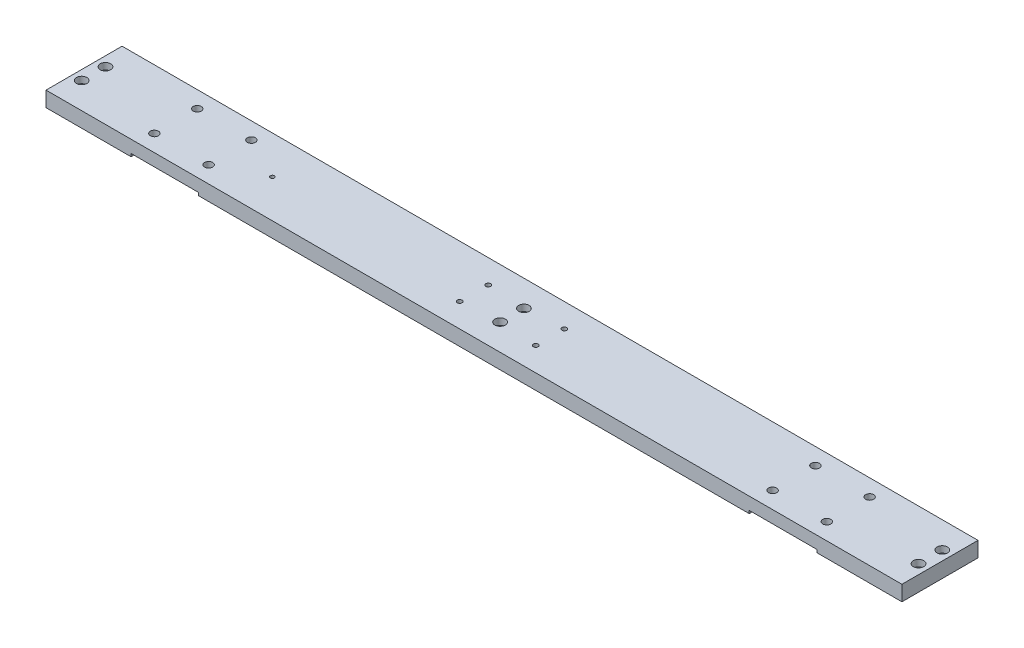
from build123d import *

# Parameters (mm, degrees)
SKETCH_1_W                = 900
SKETCH_1_H                = 80
EXTRUDE_1_DEPTH           = 16
SKETCH_2_W                = 71.098057304
SKETCH_2_H                = 80
CUT_EXTRUDE_1_DEPTH       = 3
HOLE_WIZARD_8_5_8_5_1_D   = 8.5
HOLE_WIZARD_M6_1_D        = 5
HOLE_WIZARD_1_D           = 6.6
HOLE_WIZARD_1_CBORE_D     = 11
HOLE_WIZARD_1_CBORE_DEPTH = 6.8
PATTERN_LINEAR_1_COUNT    = 3
PATTERN_LINEAR_1_PITCH    = 440
HOLE_WIZARD_M5_1_D        = 4.2


with BuildPart() as part:
    # 草图1 → 凸台-拉伸1 (new body)
    with BuildSketch(Plane(origin=(0, 0, 0), x_dir=(1, 0, 0), z_dir=(0, 1, 0))):
        Rectangle(SKETCH_1_W, SKETCH_1_H)
    extrude(amount=EXTRUDE_1_DEPTH)

    # 草图2 → 切除-拉伸1 (cut)
    with BuildSketch(Plane.XZ):
        with Locations((-325, 0)):
            Rectangle(SKETCH_2_W, SKETCH_2_H)
        with Locations((325, 0)):
            Rectangle(SKETCH_2_W, SKETCH_2_H)
    extrude(amount=-CUT_EXTRUDE_1_DEPTH, mode=Mode.SUBTRACT)

    # Ø8.5 (8.5) 直径孔1 (through all)
    with Locations(Plane(origin=(0, 16, 0), x_dir=(1, 0, 0), z_dir=(0, 1, 0))):
        with Locations((-353.5, 22.5), (-296.5, 22.5), (-353.5, -22.5), (-296.5, -22.5)):
            hole_wizard_8_5_8_5_1 = Hole(HOLE_WIZARD_8_5_8_5_1_D / 2)

    # 镜向1: Ø8.5 (8.5) 直径孔1 across plane
    add(hole_wizard_8_5_8_5_1.mirror(Plane(origin=(0, 0, 0), x_dir=(0, 0, 1), z_dir=(1, 0, 0))), mode=Mode.SUBTRACT)

    # M6 螺纹孔1 (through all)
    with Locations(Plane(origin=(0, 16, 0), x_dir=(1, 0, 0), z_dir=(0, 1, 0))):
        with Locations((-40, 15), (40, 15), (-40, -15), (40, -15)):
            Hole(HOLE_WIZARD_M6_1_D / 2)

    # 打孔尺寸(%根据)内六角圆柱头螺钉的类型1 (through all)
    with Locations(Plane(origin=(0, 16, 0), x_dir=(1, 0, 0), z_dir=(0, 1, 0))):
        with Locations((-440, 12.5), (-440, -12.5)):
            hole_wizard_1 = CounterBoreHole(HOLE_WIZARD_1_D / 2, HOLE_WIZARD_1_CBORE_D / 2, HOLE_WIZARD_1_CBORE_DEPTH)

    # 阵列(线性)1: 打孔尺寸(%根据)内六角圆柱头螺钉的类型1 ×3
    with Locations(*[(i * PATTERN_LINEAR_1_PITCH, 0, 0) for i in range(1, PATTERN_LINEAR_1_COUNT)]):
        add(hole_wizard_1, mode=Mode.SUBTRACT)

    # M5 螺纹孔1 (through all)
    with Locations(Plane(origin=(0, 16, 0), x_dir=(1, 0, 0), z_dir=(0, 1, 0))):
        with Locations((-252, 0)):
            Hole(HOLE_WIZARD_M5_1_D / 2)


solid = part.part
